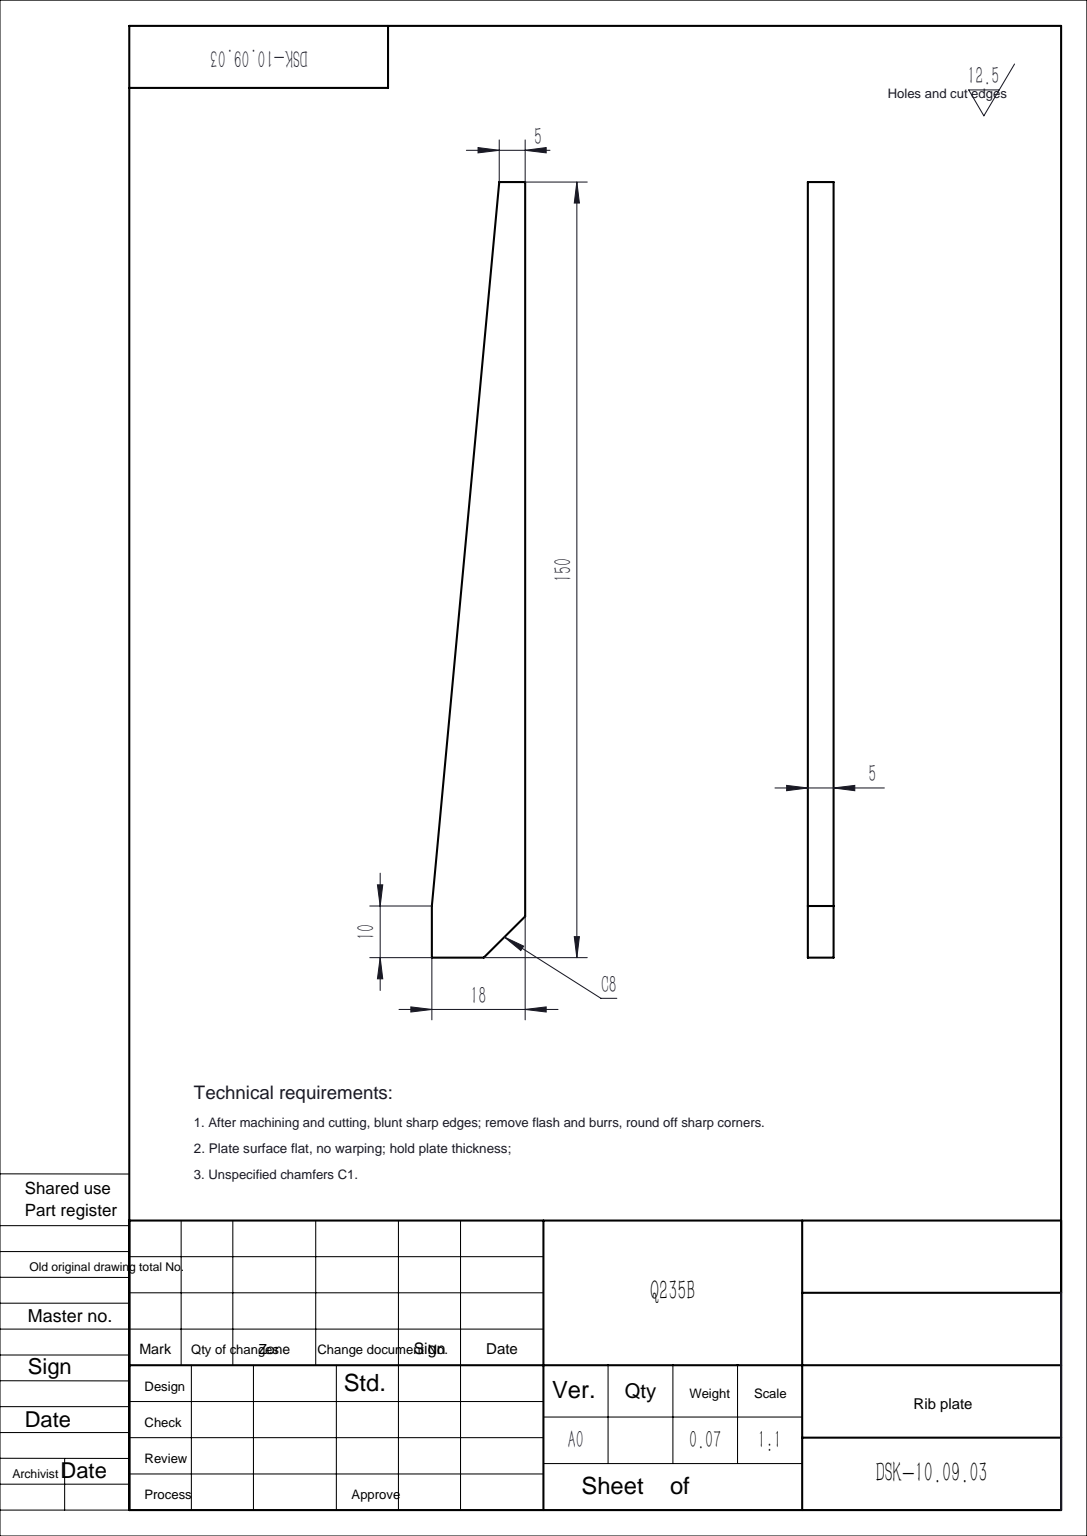
from build123d import *

# Parameters (mm, degrees)
BOSS_EXTRUDE1_DEPTH = 5


with BuildPart() as part:
    # Sketch1 → Boss-Extrude1 (new body)
    with BuildSketch(Plane.XY):
        Polygon((0, 0), (0, 10), (13, 150), (18, 150), (18, 8), (10, 0), align=None)
    extrude(amount=BOSS_EXTRUDE1_DEPTH)


solid = part.part
